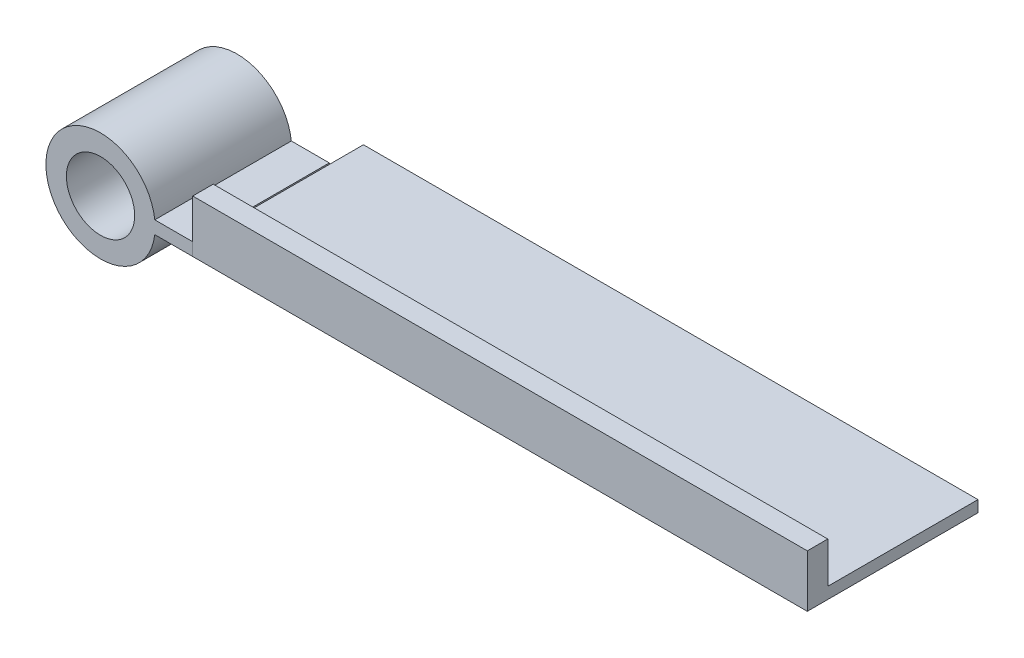
SolidWorks part; units mm, degrees
ref_plane "Front Plane" through (0, 0, 0) normal (0, 0, 1) x (1, 0, 0)
ref_plane "Top Plane" through (0, 0, 0) normal (0, 1, 0) x (1, 0, 0)
ref_plane "Right Plane" through (0, 0, 0) normal (1, 0, 0) x (0, 0, -1)
other "Configuration Table"
sketch "Sketch1" plane through (0, 0, 0) normal (0, 0, 1) x (1, 0, 0)
  circle A0 centre (0, 0) radius 5
  circle A1 centre (0, 0) radius 8
  dimension "D1" = 16
  dimension "D2" = 10
extrude "Boss-Extrude1" add sketch "Sketch1" along normal mid plane 20
sketch "Sketch3" plane through (0, 0, 0) normal (0, 0, 1) x (1, 0, 0)
  line L1 (5.5, -0.9375) -> (13.5, -0.9375)
  line L2 (5.5, -0.9375) -> (5.5, 0.9375)
  line L3 (5.5, 0.9375) -> (13.5, 0.9375)
  line L4 (13.5, -0.9375) -> (13.5, 0.9375)
  line L5 (5.5, -0.9375) -> (13.5, 0.9375) construction
  line L6 (5.5, 0.9375) -> (13.5, -0.9375) construction
  point P0 (9.5, 0)
  dimension "D1" = 5.5
  dimension "D2" = 8
extrude "Boss-Extrude2" add sketch "Sketch3" along normal mid plane 20
sketch "Sketch4" plane through (0, 0, 10) normal (0, 0, 1) x (1, 0, 0)
  line L1 (13.5, -0.9375) -> (103.5, -0.9375)
  line L2 (13.5, -0.9375) -> (13.5, 6.7377)
  line L3 (13.5, 6.7377) -> (103.5, 6.7377)
  line L4 (103.5, -0.9375) -> (103.5, 6.7377)
  dimension "D1" = 90
extrude "Boss-Extrude3" add sketch "Sketch4" against normal blind 25 separate body
sketch "Sketch5" plane through (0, 6.7377, 0) normal (0, 1, 0) x (1, 0, 0)
  line L0 (103.5, 15) -> (103.5, -10) construction
  line L1 (13.5, 15) -> (103.5, 15)
  line L2 (13.5, 15) -> (13.5, -7)
  line L3 (13.5, -7) -> (103.5, -7)
  line L4 (103.5, 15) -> (103.5, -7)
  dimension "D1" = 22
extrude "Cut-Extrude1" cut sketch "Sketch5" against normal blind 6
